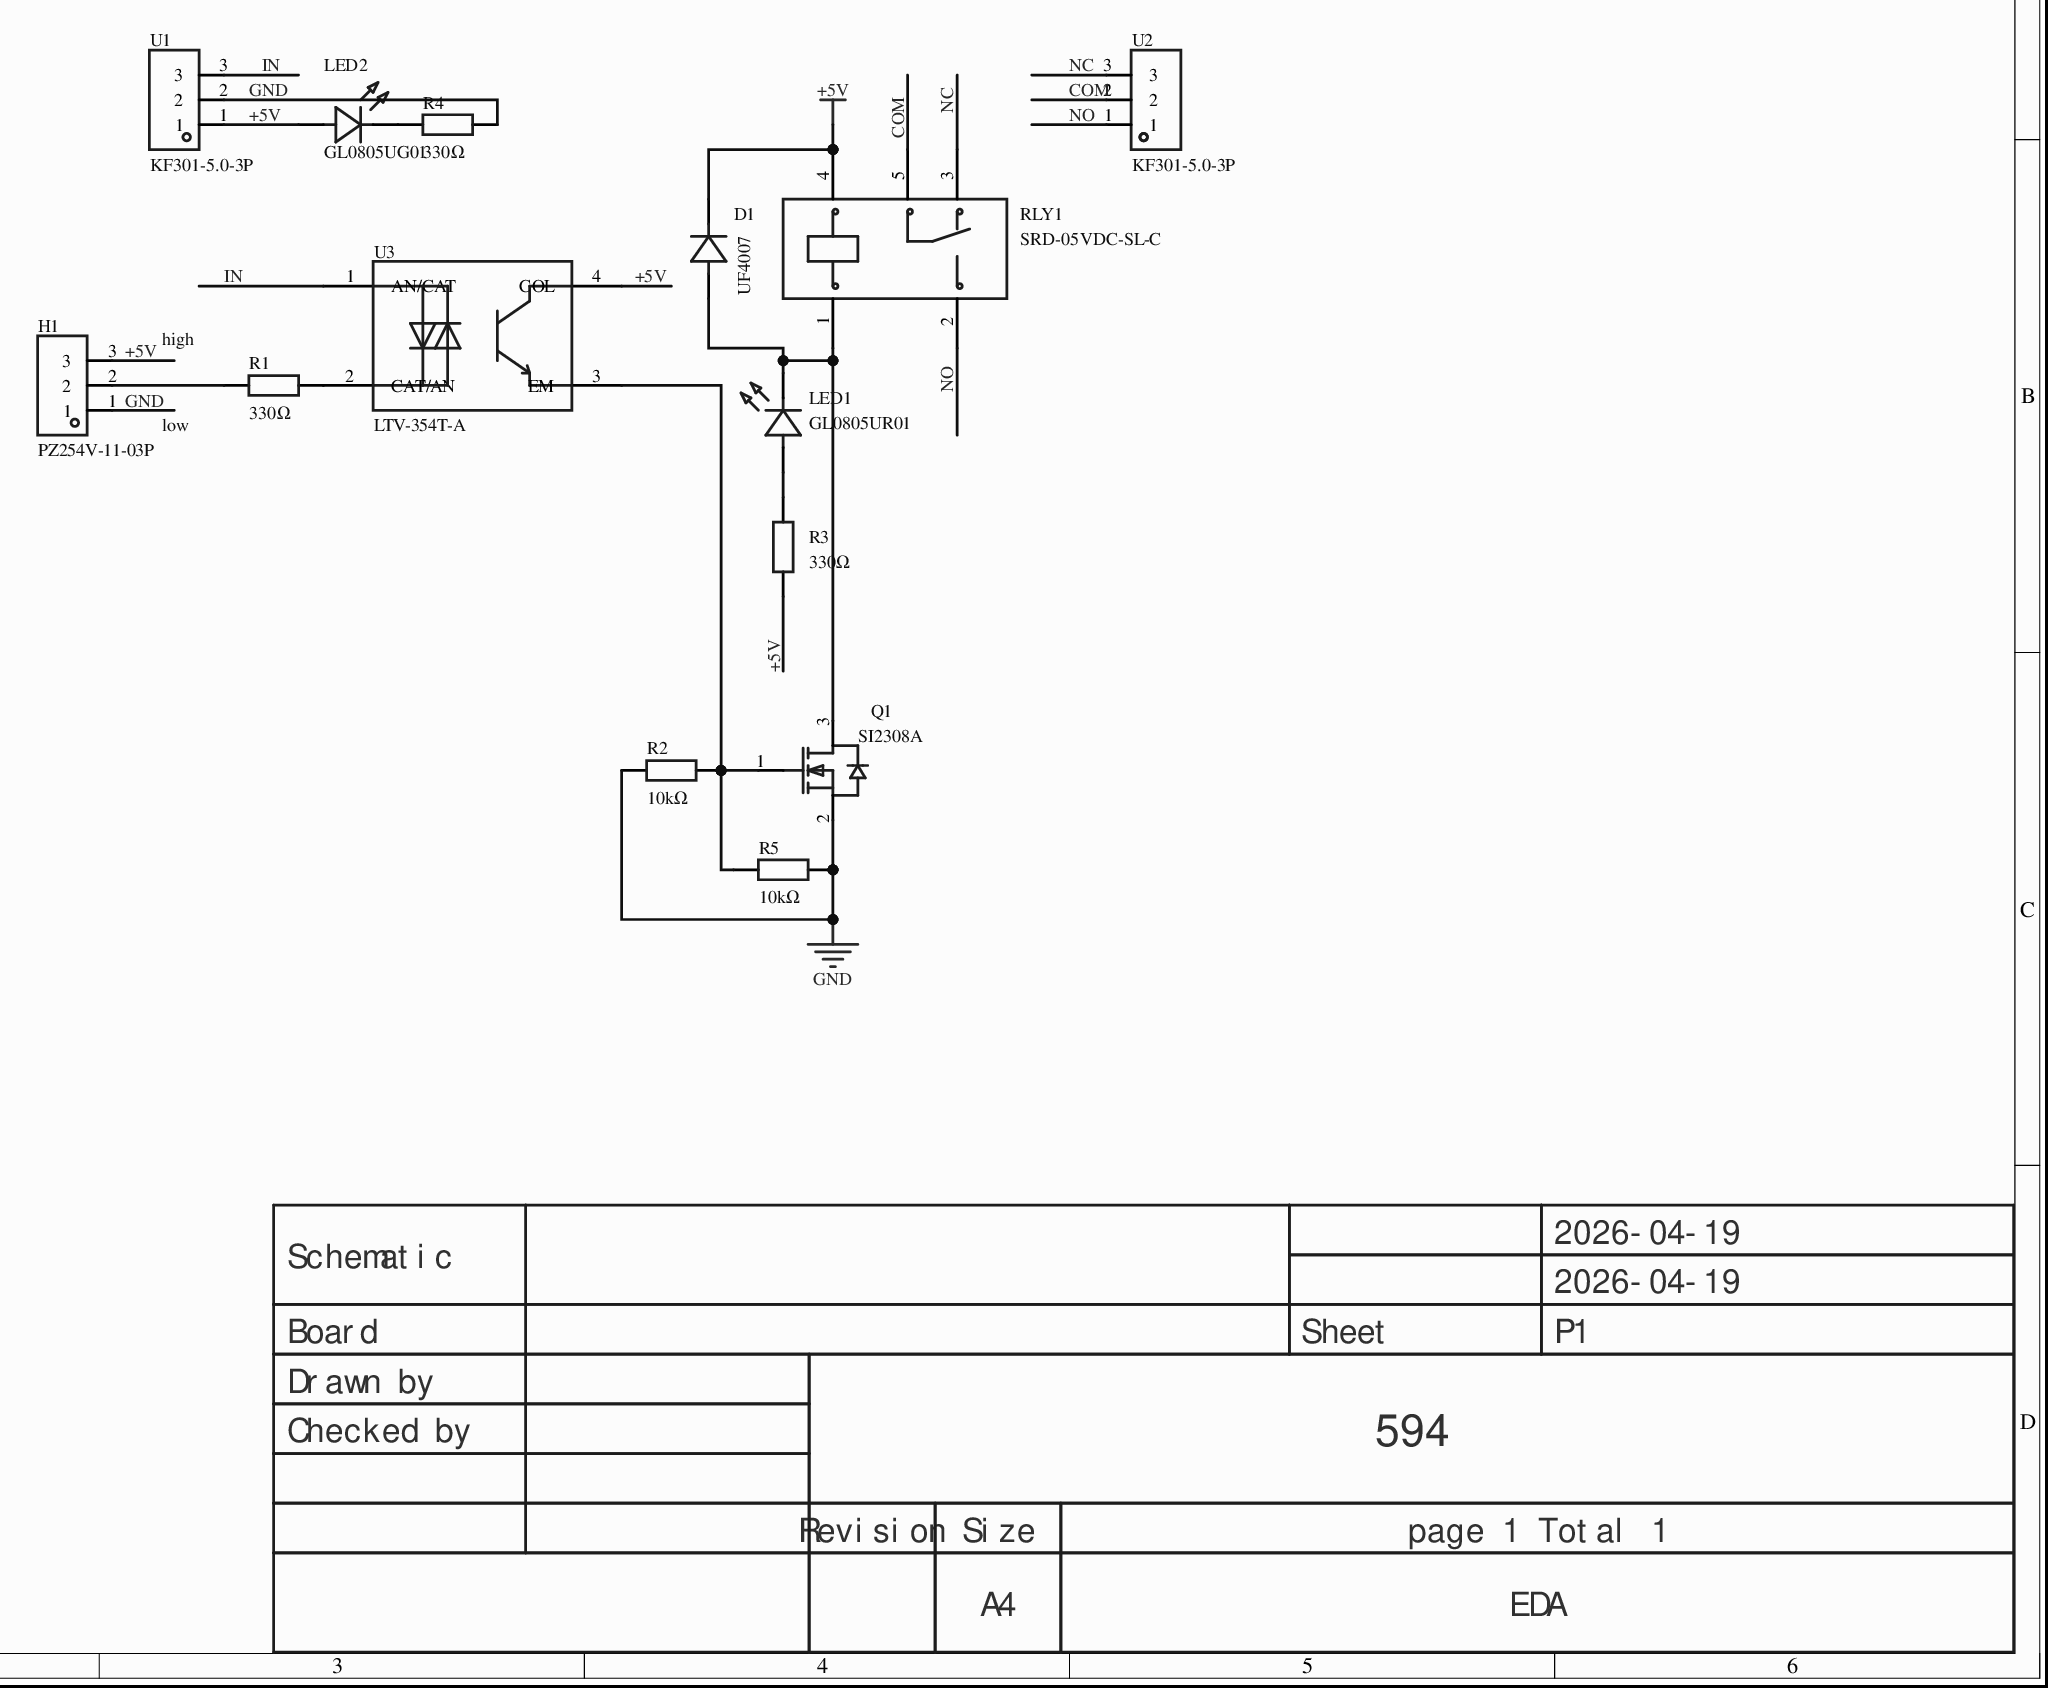
[diagram p0: MISC49931-3.schdoc]
# Altium project MISC49931-2.PrjPcb
1 sheet, 14 parts. Net scope: global (net labels, ports and power ports of the same name join across sheets).
Board file: MISC49931.pcbdoc

## Sheet MISC49931-3.schdoc
size 297 x 209 mm; Version: V1.0; @Project Name: MISC49931; @Update Date: 2026-04-19; @Create Date: 2026-04-19; @Board Name: MISC49931; @Create Time: 19:38:57; @Page Count: 1; @Page No: 1; @Schematic Name: MISC49931; @Update Time: 19:38:57; Size: A4

### Parts
D1  UF4007  [DO-41_BD2.4-L4.7-P8.70-D0.9-RD]
H1  PZ254V-11-03P  [HDR-TH_3P-P2.54-V-M_PZ254V-11-03P]
LED1  GL0805UR01  [LED0805-R-RD_RED]
LED2  GL0805UG01  [LED0805-FD_GL0805UG01]
Q1  SI2308A  [SOT-23-3_L2.9-W1.3-P1.90-LS2.4-BR]
R1  330Ω  [R0603]
R2  10kΩ  [R0603]
R3  330Ω  [R0603]
R4  330Ω  [R0603]
R5  10kΩ  [R0603]
RLY1  SRD-05VDC-SL-C  [RELAY-TH_SRD-XXVDC-XL-C]
U1  KF301-5.0-3P  [CONN-TH_3P-P5.00_KF301-5.0-3P]
U2  KF301-5.0-3P  [CONN-TH_3P-P5.00_KF301-5.0-3P]
U3  LTV-354T-A  [SOP-4_L3.9-W4.4-P2.54-LS7.0-TL]

### Nets
+5V: D1.1(K) H1.3 LED2.1(A) R3.1 RLY1.4 U1.1 U3.4(COL)
GND: H1.1 Q1.2(S) R2.1 R4.2 R5.2 U1.2
COM: RLY1.5 U2.2
IN: U1.3 U3.1(AN/CAT)
NC: RLY1.3 U2.3
NO: RLY1.2 U2.1
NetD1_2: D1.2(A) LED1.2(C) Q1.3(D) RLY1.1
NetH1_2: H1.2 R1.1
NetLED1_1: LED1.1(A) R3.2
NetLED2_2: LED2.2(C) R4.1
NetQ1_1: Q1.1(G) R2.2 R5.1 U3.3(EM)
NetR1_2: R1.2 U3.2(CAT/AN)

### Notes on the sheet
- high
- low
- 2026-04-19
- Schematic
- Board
- Sheet
- P1
- Drawn by
- Checked by
- 594
- Revision
- Size
- A4
- page 1 Total 1
- EDA

### Library data of the parts
D1 = UF4007_C960666: Diode configuration: -; forward voltage (Vf): 1.7V@1A; reverse breakdown voltage (Vr): 1kV; rectified current: 1A; reverse recovery time (Trr): 75ns;; Manufacturer: MDD(辰达半导体); 3D Model: 6de1e9b71a0d4751b4e9df530304c1a30819f05c4eef4c71ace90d822a990e87; 3D Model Transform: 374.016,94.488,0,0,0,0,0,0,-137.795; Reverse Leakage Current (Ir): 5uA@1kV; Operating Junction Temperature Range: -50℃~+150℃@(Tj); Non-Repetitive Peak Forward Surge Current: 30A; AddInBom: yes; ModelName: DO-41_D2.4-L4.7-P8.70; Symbol: UF4007_C960666; Device: UF4007_C960666; LCSC Part Name: 耐压:1kV 电流:1A 反向恢复时间：75ns; Supplier Part: C960666; Manufacturer Part: UF4007; Supplier Footprint: DO-41; JLCPCB Part Class: Extended Part; Datasheet: https://example.com/datasheet/UF4007/1039942.html; Supplier: LCSC; Diode Configuration: -; Voltage - Forward(Vf@If): 1.7V@1A; Voltage - DC Reverse(Vr): 1kV; Current - Rectified: 1A; Reverse Recovery Time (trr): 75ns; ConvertToPcb: yes; FootprintName: DO-41_BD2.4-L4.7-P8.70-D0.9-RD
H1 = PZ254V-11-03P: Pin structure: 1x3P; pitch: 2.54mm; row spacing: -; round/square pin: square pin; mounting: through-hole; rows: single row; total pins: 3P; rated current: 3A; rated voltage: 250V; mating pin length: 6mm; insulation height: 2.5mm; end connection pin length: 3mm; operating temperature: -40℃~+105℃; colour: black;; Manufacturer: XFCN(兴飞); Symbol: PZ254V-11-03P_C2937625; 3D Model: bd28a638fbd247be9398fd5d39c366ec0819f05c4eef4c71ace90d822a990e87; 3D Model Transform: 300.3931,100,0,0,0,0,0,0,-118.11; AddInBom: yes; Device: PZ254V-11-03P; LCSC Part Name: 1x3P 间距:2.54mm 方针 直插; Supplier Part: C2937625; Manufacturer Part: PZ254V-11-03P; Supplier Footprint: 插件,P=2.54mm; JLCPCB Part Class: Extended Part; Datasheet: https://example.com/datasheet/PZ254V-11-03P/3293280.html; Supplier: LCSC; Pin Structure: 1x3P; Pitch: 2.54mm; Row Spacing: -; Circluar Pins/Square Pins: Square pin; Mounting Type: Through-hole; Number of Rows: Single row; Number of Pins: 3P; Current Rating: 3A; Voltage Rating (Max): 250V; Length of Mating Pin: 6mm; Insulation Height: 2.5mm; Length of End Connection Pin: 3mm; Operating Temperature: -40℃~+105℃; Color: Black; ConvertToPcb: yes; FootprintName: HDR-TH_3P-P2.54-V-M_PZ254V-11-03P; ModelName: HDR-TH_3P-P2.54-V-M_PZ254V-11-03P
LED1 = GL0805UR01: Light colour: red; forward voltage (Vf): 2.1V; forward current: 10mA; wavelength: 618nm~624nm; diode configuration: single diode; lens colour: clear lens; luminous intensity: 100mcd; viewing angle: 120°; tape and reel: top mount; operating temperature: -40℃~+85℃;; Manufacturer: Guiguang light(桂光光电); 3D Model: f010e90d36544999ab4e363fdba5b4900819f05c4eef4c71ace90d822a990e87; 3D Model Transform: 78.74,49.21644,0,0,0,0,0,0,0; AddInBom: yes; Symbol: GL0805UR01; Device: GL0805UR01; LCSC Part Name: 0805 红灯 高亮; Supplier Part: C51933307; Manufacturer Part: GL0805UR01; Supplier Footprint: 0805; JLCPCB Part Class: Extended Part; Datasheet: https://example.com/datasheet/GL0805UR01/54646003.html; Supplier: LCSC; Illumination Color: Red; Voltage - Forward(Vf): 2.1V; Forward Current: 10mA; Wavelength - Dominant: 618nm~624nm; Diode Configuration: Single diode; Lens Color: Clear lens; Luminous Intensity: 100mcd; Viewing Angle: 120°; Mounting Style: Top mount; Operating Temperature: -40℃~+85℃; ConvertToPcb: yes; FootprintName: LED0805-R-RD_RED; ModelName: LED0805-R-RD_RED
LED2 = GL0805UG01: Base type: -; light colour: emerald green; forward voltage (Vf): 3.1V; power: -; forward current: 5mA; wavelength: 510nm~531nm; diode configuration: single diode; lens colour: clear lens; colour temperature: -; luminous intensity: 299mcd; viewing angle: 120°; tape and reel: top mount; operating temperature: -40℃~+85℃;; Manufacturer: Guiguang light(桂光光电); AddInBom: yes; Symbol: GL0805UG01; Device: GL0805UG01; LCSC Part Name: 0805 翠绿 高亮; Supplier Part: C51933308; Manufacturer Part: GL0805UG01; Supplier Footprint: 0805; JLCPCB Part Class: Extended Part; Datasheet: https://example.com/datasheet/GL0805UG01/54646004.html; Supplier: LCSC; Lamp Holder Type: -; Illumination Color: Emerald green; Voltage - Forward(Vf): 3.1V; Power(Watts): -; Forward Current: 5mA; Wavelength - Dominant: 510nm~531nm; Peak Wavelength: -; Diode Configuration: Single diode; Lens Color: Clear lens; Color Temperature: -; Luminous Intensity: 299mcd; Viewing Angle: 120°; Mounting Style: Top mount; Operating Temperature: -40℃~+85℃; ConvertToPcb: yes; FootprintName: LED0805-FD_GL0805UG01
Q1 = SI2308A: Quantity: 1 N-channel; drain-source voltage (Vdss): 60V; continuous drain current (Id): 3A; on-resistance (RDS(on)): 80mΩ@10V; 95mΩ@4.5V; power dissipation (Pd): 1.25W; threshold voltage (Vgs(th)): 3V@250uA;; Manufacturer: UMW(友台半导体); 3D Model: c62791f0466c4ae2a892c056b845b0ca0819f05c4eef4c71ace90d822a990e87; 3D Model Transform: 98.425,114.173,0,180,0,0,0.0005,-0.0005,0; Gate Charge(Qg): 4.8nC@10V; Input Capacitance(Ciss): 240pF; Reverse Transfer Capacitance (Crss@Vds): 15pF; Output Capacitance(Coss): 50pF; AddInBom: yes; ModelName: SOT-23-3P_L2.9-W1.3-H1.0-LS2.4-P0.95; Symbol: SI2308A; Device: SI2308A; LCSC Part Name: 1个N沟道 耐压:60V 电流:3A; Supplier Part: C347491; Manufacturer Part: SI2308A; Supplier Footprint: SOT-23; JLCPCB Part Class: Extended Part; Datasheet: https://example.com/datasheet/SI2308A/324151.html; Supplier: LCSC; Number: 1 N-channel; Drain to Source Voltage: 60V; Current - Continuous Drain(Id): 3A; RDS(on): 80mΩ@10V; 95mΩ@4.5V; Pd - Power Dissipation: 1.25W; Gate Threshold Voltage (Vgs(th)): 3V@250uA; Operating Temperature: -40℃~+150℃; Type: N-channel; ConvertToPcb: yes; FootprintName: SOT-23-3_L2.9-W1.3-P1.90-LS2.4-BR
R1 R3 R4 = 0603WAF3300T5E: Resistor type: thick film resistor; resistance: 330Ω; tolerance: ±1%; power: 100mW; max working voltage: 75V; temperature coefficient: ±100ppm/℃;; Manufacturer: UNI-ROYAL(厚声); 3D Model: fc143cca1e79419f9cd78b61e9279f080819f05c4eef4c71ace90d822a990e87; 3D Model Transform: 31.8897,63.7794,0,90,0,0,0,0,0; AddInBom: yes; Symbol: 0603WAF3300T5E; Device: 0603WAF3300T5E; LCSC Part Name: 330Ω ±1% 100mW 厚膜电阻; Supplier Part: C23138; Manufacturer Part: 0603WAF3300T5E; Supplier Footprint: 0603; JLCPCB Part Class: Basic Part; Datasheet: https://example.com/upload/public/pdf/source/20200306/C422600_1E6D84923E4A46A82E41ADD87F860B5C.pdf; Supplier: LCSC; Type: Thick film resistor; Value: 330Ω; Tolerance: ±1%; Power(Watts): 100mW; Overload Voltage (Max): 75V; Temperature Coefficient: ±100ppm/℃; Operating Temperature Range: -55℃~+155℃; ConvertToPcb: yes; FootprintName: R0603; ModelName: R0603
R2 R5 = 0603WAJ0103T5E: Resistor type: thick film resistor; resistance: 10kΩ; tolerance: ±5%; power: 100mW; max working voltage: 75V; temperature coefficient: ±100ppm/℃;; Manufacturer: UNI-ROYAL(厚声); 3D Model: fc143cca1e79419f9cd78b61e9279f080819f05c4eef4c71ace90d822a990e87; 3D Model Transform: 31.8897,63.7794,0,90,0,0,0,0,0; AddInBom: yes; Symbol: 0603WAJ0103T5E; Device: 0603WAJ0103T5E; LCSC Part Name: 10kΩ ±5% 100mW 厚膜电阻; Supplier Part: C15401; Manufacturer Part: 0603WAJ0103T5E; Supplier Footprint: 0603; JLCPCB Part Class: Extended Part; Datasheet: https://example.com/upload/public/pdf/source/20200306/C422600_1E6D84923E4A46A82E41ADD87F860B5C.pdf; Supplier: LCSC; Type: Thick film resistor; Value: 10kΩ; Tolerance: ±5%; Power(Watts): 100mW; Overload Voltage (Max): 75V; Temperature Coefficient: ±100ppm/℃; Operating Temperature Range: -55℃~+155℃; ConvertToPcb: yes; FootprintName: R0603; ModelName: R0603
RLY1 = SRD-05VDC-SL-C: Coil voltage: 5V; contact form: changeover 1C (SPDT); contact rating (resistive load): -; max switching voltage: 250V@AC; max switching current: 15A;; Manufacturer: 松乐; 3D Model: d0eda9b8bf8746d18ae810ab88dc78e70819f05c4eef4c71ace90d822a990e87; 3D Model Transform: 755.904,622.4397,0,0,0,0,34.882,0,-118.11; Contact Form: Changeover contact: 1C (SPDT); Coil Rated Power: 360mW; Coil Type: Non-polarised, single coil; Coil Resistance: 70Ω; Contact Resistance: 100mΩ; Operate Time: 10ms; AddInBom: yes; ModelName: RELAY-TH_L19.2-W15.6-H15.8; Symbol: SRD-05VDC-SL-C; Device: SRD-05VDC-SL-C; LCSC Part Name: 蓝色 单组转换型继电器; Supplier Part: C35449; Manufacturer Part: SRD-05VDC-SL-C; Supplier Footprint: 插件,15.6x19.2mm; JLCPCB Part Class: Extended Part; Datasheet: https://example.com/datasheet/SRD-05VDC-SL-C/36422.html; Supplier: LCSC; Coil Voltage: 5V; Number of Pins: 5; Contact Rating: -; Switching Voltage(Max): 250V@AC; Switching Current(Max): 15A; Release Time: 10ms; ConvertToPcb: yes; FootprintName: RELAY-TH_SRD-XXVDC-XL-C
U1 U2 = KF301-5.0-3P: Structure: 1x3P; pitch: 5mm; colour: blue; mounting: through-hole; rows: 1; pins per row: 3; rated current: 17A; rated voltage: 250V; wire gauge - AWG: 14~22; wire gauge - mm²: 1.5; operating temperature: -30℃~+120℃;; Manufacturer: KEFA(科发); 3D Model: 7090fd1e13c24e5e88660dd73c4524570819f05c4eef4c71ace90d822a990e87; 3D Model Transform: 606.298,303.149,0,0,0,0,7.874,5.906,-169.291; Number of PINs Per Row: 3; Wire Gauge - mm2: 1.5; AddInBom: yes; Symbol: KF301-5.0-3P; Device: KF301-5.0-3P; LCSC Part Name: 1x3P 5mm 直插 排数:1 每排P数:3; Supplier Part: C474882; Manufacturer Part: KF301-5.0-3P; Supplier Footprint: 插件,P=5mm; JLCPCB Part Class: Extended Part; Datasheet: https://example.com/datasheet/KF301-5.0-3P/481500.html; Supplier: LCSC; Number of Positions or Pins: 1x3P; Pitch: 5mm; Color: Blue; Mounting Type: Through-hole; Number of Pins: 3P; Number of Rows: 1; Current Rating: 17A; Voltage Rating (Max): 250V; Wire Gauge - AWG: 14~22; Operating Temperature: -30℃~+120℃; ConvertToPcb: yes; FootprintName: CONN-TH_3P-P5.00_KF301-5.0-3P; ModelName: CONN-TH_3P-P5.00_KF301-5.0-3P
U3 = LTV-354T-A: Input type: AC,DC; forward voltage (Vf): 1.2V; output current: 50mA; isolation voltage (Vrms): 3.75kV; reverse breakdown voltage (Vr): -; load voltage: 35V; output channels: 1; collector-emitter saturation voltage (VCE(sat)): 100mV@20mA,1mA;; Manufacturer: LITEON(光宝); 3D Model: ddaef38cfbc4419f8552fc0322b021000819f05c4eef4c71ace90d822a990e87; 3D Model Transform: 157.48,275.824,0,270,0,0,0,0,0; Input type: AC,DC; Output Type: Phototransistor; Number of Outputs: 1; Rise time: 4us; Fall time: 3us; Current Transfer Ratio (CTR) Minimum: 20%; Current Transfer Ratio (CTR) Maximum/Saturation Value: 400%; Total Power Dissipation(Pd): 170mW; AddInBom: yes; ModelName: SOP-4_L4.0-W4.4-H2.1-LS7.0-P2.54; Symbol: LTV-354T-A; Device: LTV-354T-A; LCSC Part Name: AC,DC输入 隔离电压(rms):3750V; Supplier Part: C10802; Manufacturer Part: LTV-354T-A; Supplier Footprint: SOP-4-2.54mm; JLCPCB Part Class: Extended Part; Datasheet: https://example.com/datasheet/LTV-354T-A/11348.html; Supplier: LCSC; Voltage - Forward(Vf): 1.2V; Output Current: 50mA; Isolation Voltage(Vrms): 3.75kV; Reverse Voltage: -; Load Voltage: 35V; Vce Saturation(VCE(sat)): 100mV@20mA,1mA; Operating Temperature: -55℃~+100℃; Forward Current(If): 50mA; ConvertToPcb: yes; FootprintName: SOP-4_L3.9-W4.4-P2.54-LS7.0-TL